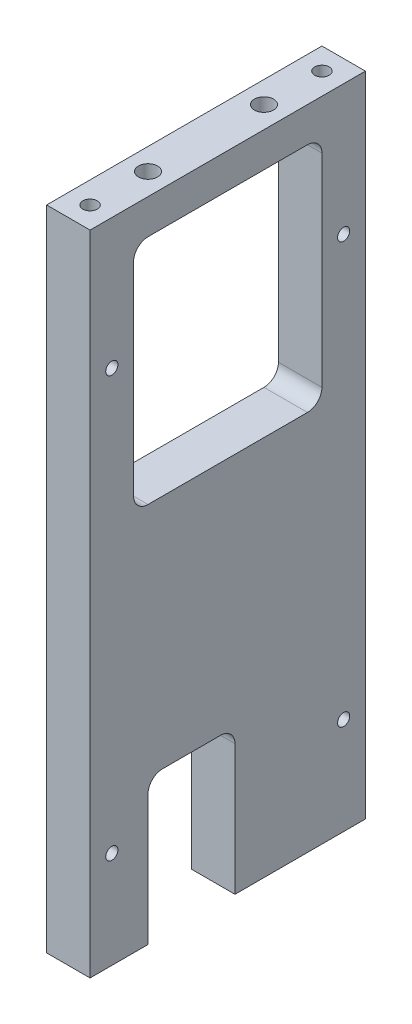
from build123d import *

# Parameters (mm, degrees)
SKETCH1_W                  = 95
SKETCH1_H                  = 223.5
BOSS_EXTRUDE1_DEPTH        = 15
CUT_EXTRUDE1_DEPTH         = 123.349141803
M6_CLEARANCE_HOLE1_D       = 6.6
M6_CLEARANCE_HOLE1_DEPTH   = 19.75
M6_CLEARANCE_HOLE1_TIP     = 1.982840043
M6_TAPPED_HOLE1_D          = 5
M6_TAPPED_HOLE1_DEPTH      = 15
M6_TAPPED_HOLE1_TIP        = 1.502151548
F_5_0MM_BLIND_HOLE_1_D     = 5
F_5_0MM_BLIND_HOLE_1_DEPTH = 8
F_5_0MM_BLIND_HOLE_1_TIP   = 1.502151548
F_5_0MM_BLIND_HOLE_2_D     = 5
F_5_0MM_BLIND_HOLE_2_DEPTH = 8
F_5_0MM_BLIND_HOLE_2_TIP   = 1.502151548
M5_TAPPED_HOLE1_D          = 4.2
M5_TAPPED_HOLE1_DEPTH      = 12.4
M5_TAPPED_HOLE1_TIP        = 1.2618073


with BuildPart() as part:
    # Sketch1 → Boss-Extrude1 (new body)
    with BuildSketch(Plane(origin=(0, 0, 0), x_dir=(0, 0, -1), z_dir=(1, 0, 0))):
        Rectangle(SKETCH1_W, SKETCH1_H)
    extrude(amount=BOSS_EXTRUDE1_DEPTH)

    # Sketch2 → Cut-Extrude1 (cut, through all)
    with BuildSketch(Plane.ZY):
        with BuildLine():
            Line((22.5, -61.75), (2.5, -61.75))
            ThreePointArc((2.5, -61.75), (-1.035533906, -63.214466094), (-2.5, -66.75))
            Line((-2.5, -66.75), (-2.5, -111.75))
            Line((-2.5, -111.75), (27.5, -111.75))
            Line((27.5, -111.75), (27.5, -66.75))
            ThreePointArc((27.5, -66.75), (26.035533906, -63.214466094), (22.5, -61.75))
        make_face()
        with BuildLine():
            Line((-27.5, 19.75), (27.5, 19.75))
            ThreePointArc((27.5, 19.75), (31.035533906, 21.214466094), (32.5, 24.75))
            Line((32.5, 24.75), (32.5, 94.75))
            ThreePointArc((32.5, 94.75), (31.035533906, 98.285533906), (27.5, 99.75))
            Line((27.5, 99.75), (-27.5, 99.75))
            ThreePointArc((-27.5, 99.75), (-31.035533906, 98.285533906), (-32.5, 94.75))
            Line((-32.5, 94.75), (-32.5, 24.75))
            ThreePointArc((-32.5, 24.75), (-31.035533906, 21.214466094), (-27.5, 19.75))
        make_face()
    extrude(amount=-CUT_EXTRUDE1_DEPTH, mode=Mode.SUBTRACT)

    # M6 Clearance Hole1
    with Locations(Plane(origin=(0, 111.75, 0), x_dir=(1, 0, 0), z_dir=(0, 1, 0))):
        with Locations((7.5, -20), (7.5, 20)):
            Hole(M6_CLEARANCE_HOLE1_D / 2, depth=M6_CLEARANCE_HOLE1_DEPTH)
            with Locations((0, 0, -(M6_CLEARANCE_HOLE1_DEPTH + M6_CLEARANCE_HOLE1_TIP / 2))):  # 118° drill point
                Cone(0, M6_CLEARANCE_HOLE1_D / 2, M6_CLEARANCE_HOLE1_TIP, mode=Mode.SUBTRACT)

    # M6 Tapped Hole1
    with Locations(Plane(origin=(0, -111.75, 0), x_dir=(-1, 0, 0), z_dir=(0, -1, 0))):
        with Locations((-7.5, -40), (-7.5, 40)):
            Hole(M6_TAPPED_HOLE1_D / 2, depth=M6_TAPPED_HOLE1_DEPTH)
            with Locations((0, 0, -(M6_TAPPED_HOLE1_DEPTH + M6_TAPPED_HOLE1_TIP / 2))):  # 118° drill point
                Cone(0, M6_TAPPED_HOLE1_D / 2, M6_TAPPED_HOLE1_TIP, mode=Mode.SUBTRACT)

    # Ø5.0mm blind hole 1
    with Locations(Plane(origin=(0, -111.75, 0), x_dir=(-1, 0, 0), z_dir=(0, -1, 0))):
        with Locations((-7.5, 10)):
            Hole(F_5_0MM_BLIND_HOLE_1_D / 2, depth=F_5_0MM_BLIND_HOLE_1_DEPTH)
            with Locations((0, 0, -(F_5_0MM_BLIND_HOLE_1_DEPTH + F_5_0MM_BLIND_HOLE_1_TIP / 2))):  # 118° drill point
                Cone(0, F_5_0MM_BLIND_HOLE_1_D / 2, F_5_0MM_BLIND_HOLE_1_TIP, mode=Mode.SUBTRACT)

    # Ø5.0mm blind hole 2
    with Locations(Plane(origin=(0, 111.75, 0), x_dir=(1, 0, 0), z_dir=(0, 1, 0))):
        with Locations((7.5, -40), (7.5, 40)):
            Hole(F_5_0MM_BLIND_HOLE_2_D / 2, depth=F_5_0MM_BLIND_HOLE_2_DEPTH)
            with Locations((0, 0, -(F_5_0MM_BLIND_HOLE_2_DEPTH + F_5_0MM_BLIND_HOLE_2_TIP / 2))):  # 118° drill point
                Cone(0, F_5_0MM_BLIND_HOLE_2_D / 2, F_5_0MM_BLIND_HOLE_2_TIP, mode=Mode.SUBTRACT)

    # M5 Tapped Hole1
    with Locations(Plane(origin=(15, 0, 0), x_dir=(0, 0, -1), z_dir=(1, 0, 0))):
        with Locations((40, 66.75), (-40, 66.75), (40, -78.25), (-40, -78.25)):
            Hole(M5_TAPPED_HOLE1_D / 2, depth=M5_TAPPED_HOLE1_DEPTH)
            with Locations((0, 0, -(M5_TAPPED_HOLE1_DEPTH + M5_TAPPED_HOLE1_TIP / 2))):  # 118° drill point
                Cone(0, M5_TAPPED_HOLE1_D / 2, M5_TAPPED_HOLE1_TIP, mode=Mode.SUBTRACT)


solid = part.part
